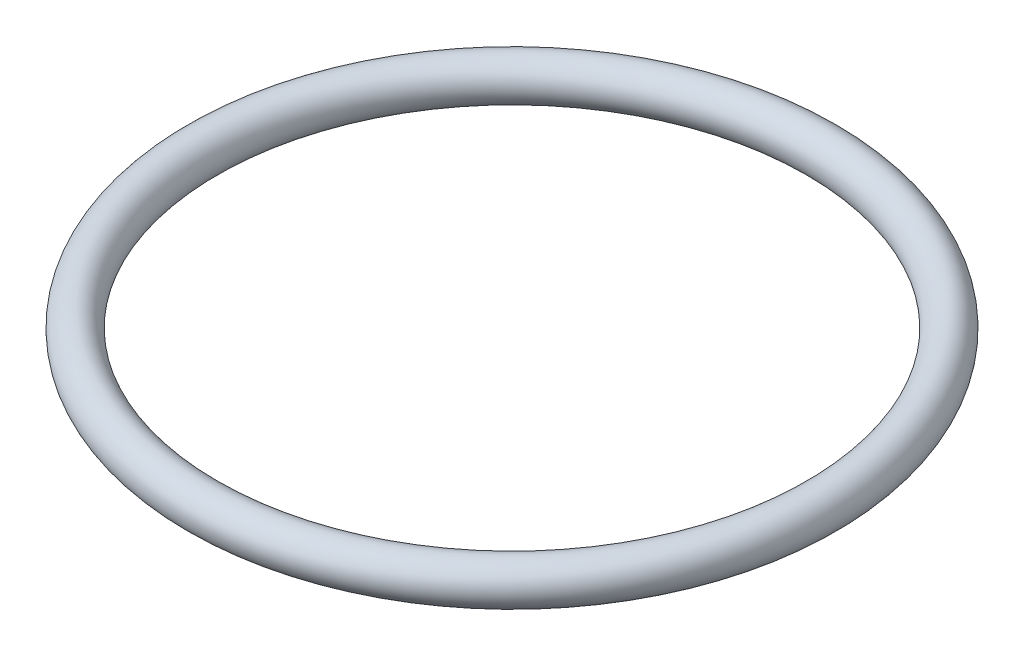
SolidWorks part; units mm, degrees
ref_plane "前视基准面" through (0, 0, 0) normal (0, 0, 1) x (1, 0, 0)
ref_plane "上视基准面" through (0, 0, 0) normal (0, 1, 0) x (1, 0, 0)
ref_plane "右视基准面" through (0, 0, 0) normal (1, 0, 0) x (0, 0, -1)
sketch "草图1" plane through (0, 0, 0) normal (0, 0, 1) x (1, 0, 0)
  line L0 (0, 0) -> (0, 3.5724) construction
  circle A0 centre (-11.25, 0) radius 0.75
  dimension "D1" = 1.5
  dimension "D2" = 22.5
revolve "旋转1" add sketch "草图1" angle 360 about L0
sketch "草图2" plane through (0, 0, 0) normal (0, 1, 0) x (1, 0, 0)
  circle A0 centre (0, 0) radius 11.1682
